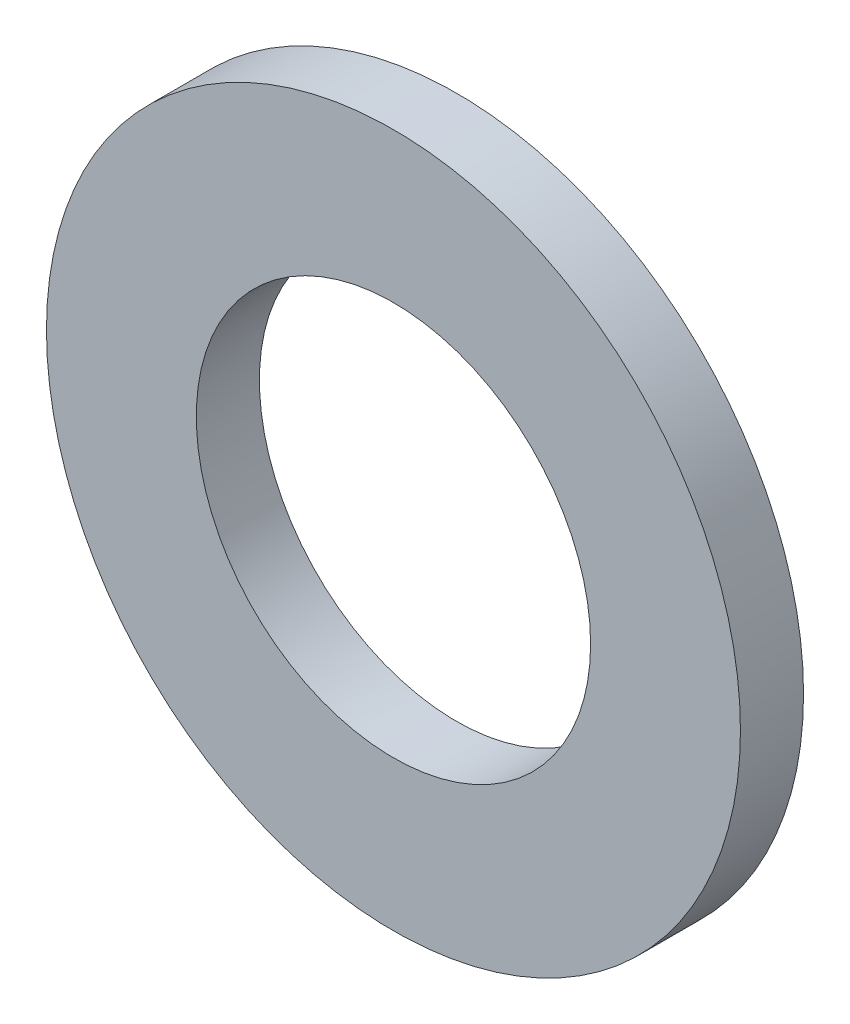
SolidWorks part; units mm, degrees
ref_plane "前视基准面" through (0, 0, 0) normal (0, 0, 1) x (1, 0, 0)
ref_plane "上视基准面" through (0, 0, 0) normal (0, 1, 0) x (1, 0, 0)
ref_plane "右视基准面" through (0, 0, 0) normal (1, 0, 0) x (0, 0, -1)
sketch "尺寸草图" plane through (0, 0, 0) normal (0, 0, 1) x (1, 0, 0)
  line L0 (0, 0) -> (4, 0) construction
  circle A0 centre (0, 0) radius 22
  circle A1 centre (0, 0) radius 12.5
  dimension "d2" = 44
  dimension "d1" = 25
  dimension "h" = 4
extrude "拉伸1" add sketch "尺寸草图" along normal blind 4
